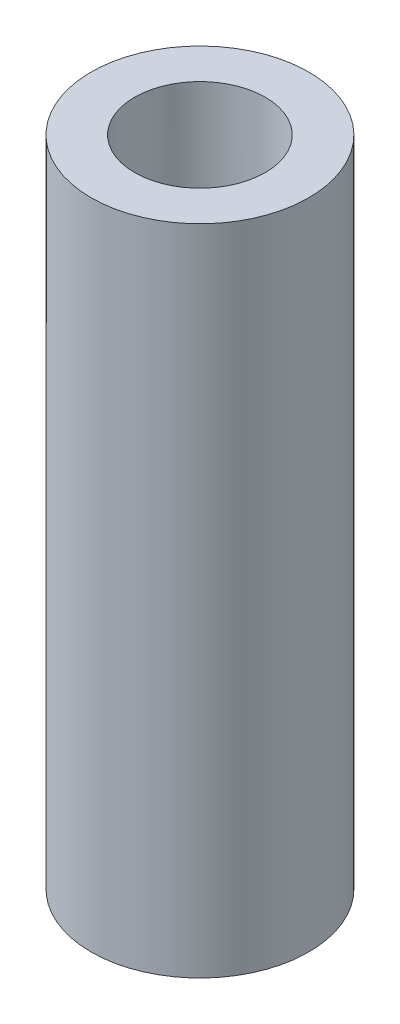
SolidWorks part; units mm, degrees
material "6061-T6 (SS)"
ref_plane "Front Plane" through (0, 0, 0) normal (0, 0, 1) x (1, 0, 0)
ref_plane "Top Plane" through (0, 0, 0) normal (0, 1, 0) x (1, 0, 0)
ref_plane "Right Plane" through (0, 0, 0) normal (1, 0, 0) x (0, 0, -1)
sketch "Sketch1" plane through (0, 0, 0) normal (0, 1, 0) x (1, 0, 0)
  circle A0 centre (0, 0) radius 2.5
  circle A1 centre (0, 0) radius 1.5
  dimension "D1" = 5
  dimension "D2" = 3
extrude "Boss-Extrude1" add sketch "Sketch1" along normal blind 15
cosmetic thread "Cosmetic Thread1" parameters "D1"=5, "D2"=4
sketch "Sketch2" plane through (0, 0, 0) normal (0, -1, 0) x (1, 0, 0)
  circle A0 centre (0, 0) radius 1.5
  circle A1 centre (0, 0) radius 0.5
  dimension "D1" = 1
extrude "Boss-Extrude2" add sketch "Sketch2" against normal blind 2
